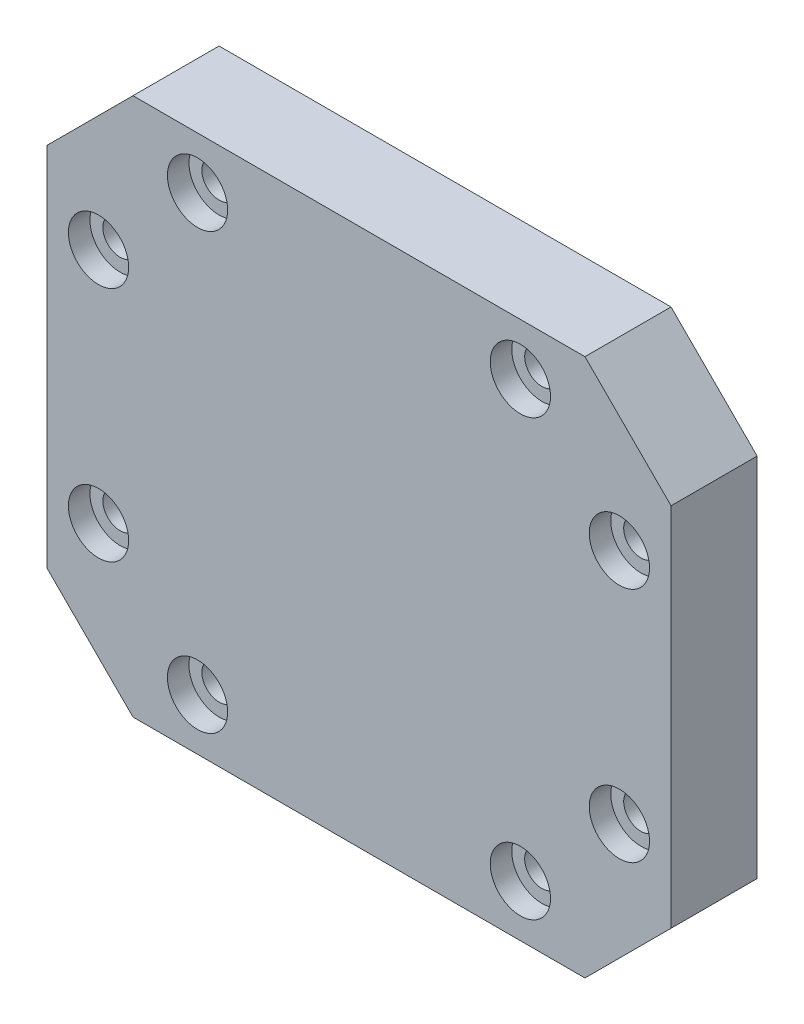
SolidWorks part; units mm, degrees
ref_plane "前视基准面" through (0, 0, 0) normal (0, 0, 1) x (1, 0, 0)
ref_plane "上视基准面" through (0, 0, 0) normal (0, 1, 0) x (1, 0, 0)
ref_plane "右视基准面" through (0, 0, 0) normal (1, 0, 0) x (0, 0, -1)
sketch "草图1" plane through (0, 0, 0) normal (0, 0, 1) x (1, 0, 0)
  line L1 (-72.5, -62.5) -> (72.5, -62.5)
  line L2 (-72.5, -62.5) -> (-72.5, 62.5)
  line L3 (-72.5, 62.5) -> (72.5, 62.5)
  line L4 (72.5, -62.5) -> (72.5, 62.5)
  line L5 (-72.5, -62.5) -> (72.5, 62.5) construction
  line L6 (-72.5, 62.5) -> (72.5, -62.5) construction
  point P0 (0, 0)
  dimension "D1" = 145
  dimension "D2" = 125
extrude "凸台-拉伸1" add sketch "草图1" along normal blind 20
chamfer "倒角1" distance 20 angle 45 4 edges at (-72.5, -62.5, 10) (72.5, -62.5, 10) (72.5, 62.5, 10) (-72.5, 62.5, 10)
sketch "草图2" plane through (0, 0, 20) normal (0, 0, 1) x (1, 0, 0)
  line L0 (52.5, 62.5) -> (-52.5, 62.5) construction
  line L1 (-72.5, 42.5) -> (-72.5, -42.5) construction
  line L2 (72.5, -42.5) -> (72.5, 42.5) construction
  line L3 (-52.5, -62.5) -> (52.5, -62.5) construction
  circle A0 centre (-37.5, 50.5) radius 7
  circle A1 centre (37.5, 50.5) radius 7
  circle A2 centre (-60.5, 27.5) radius 7
  circle A3 centre (-60.5, -27.5) radius 7
  circle A4 centre (-37.5, -50.5) radius 7
  circle A5 centre (37.5, -50.5) radius 7
  circle A6 centre (60.5, 27.5) radius 7
  circle A7 centre (60.5, -27.5) radius 7
extrude "切除-拉伸1" cut sketch "草图2" against normal blind 5
sketch "草图3" plane through (0, 0, 15) normal (0, 0, 1) x (1, 0, 0)
  circle A0 centre (-37.5, 50.5) radius 4
  circle A1 centre (-60.5, 27.5) radius 4
  circle A2 centre (-60.5, -27.5) radius 4
  circle A3 centre (-37.5, -50.5) radius 4
  circle A4 centre (37.5, 50.5) radius 4
  circle A5 centre (60.5, 27.5) radius 4
  circle A6 centre (60.5, -27.5) radius 4
  circle A7 centre (37.5, -50.5) radius 4
  dimension "D1" = 8
extrude "切除-拉伸2" cut sketch "草图3" against normal up to next
sketch "草图4" plane through (0, 0, 0) normal (0, 0, -1) x (-1, 0, 0)
  line L1 (19, 15.5) -> (-19, 15.5)
  line L2 (19, 15.5) -> (19, -15.5)
  line L3 (19, -15.5) -> (-19, -15.5)
  line L4 (-19, 15.5) -> (-19, -15.5)
  line L5 (19, 15.5) -> (-19, -15.5) construction
  line L6 (19, -15.5) -> (-19, 15.5) construction
  point P0 (0, 0)
  dimension "D1" = 31
  dimension "D2" = 38
extrude "切除-拉伸3" cut sketch "草图4" against normal blind 1.5
sketch "草图5" plane through (0, 0, 0) normal (0, 0, -1) x (-1, 0, 0)
  circle A0 centre (19, -15.5) radius 2.5
  circle A1 centre (-19, -15.5) radius 2.5
  circle A2 centre (-19, 15.5) radius 2.5
  circle A3 centre (19, 15.5) radius 2.5
  dimension "D1" = 5
extrude "切除-拉伸4" cut sketch "草图5" against normal blind 1.5
equation "\"D5@草图2\"=\"D4@草图2\""
equation "\"D6@草图2\"=\"D4@草图2\""
equation "\"D7@草图2\"=\"D2@草图2\""
equation "\"D8@草图2\"=\"D2@草图2\""
equation "\"D9@草图2\"=\"D2@草图2\""
equation "\"D3@草图2\"=\"D4@草图2\""
